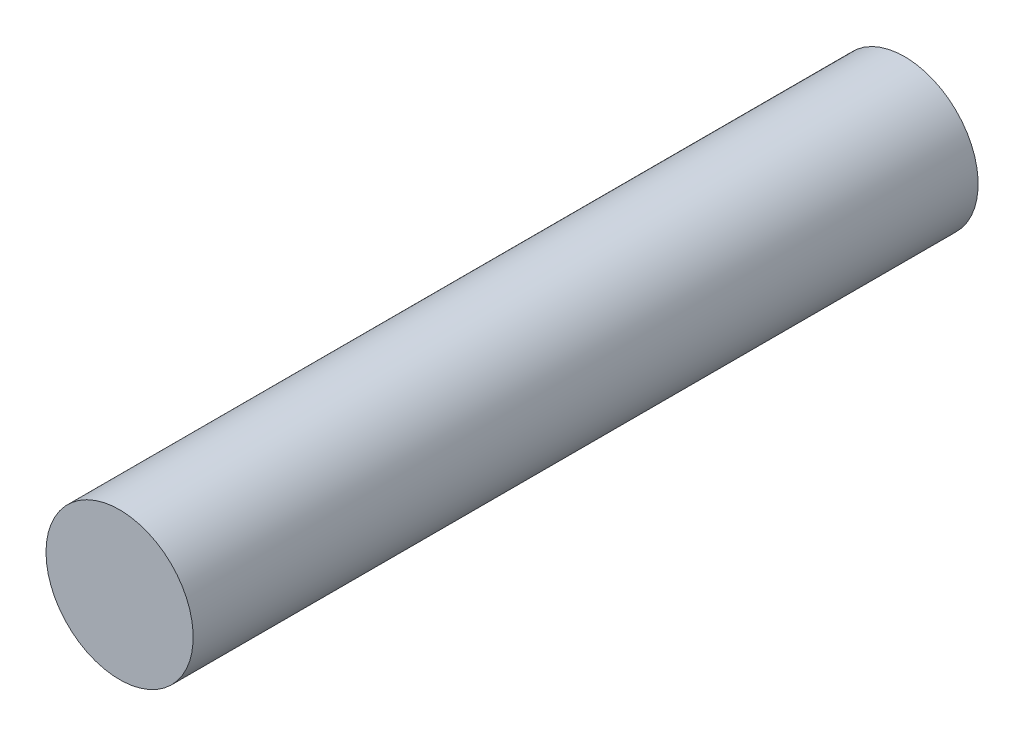
SolidWorks part; units mm, degrees
ref_plane "Front Plane" through (0, 0, 0) normal (0, 0, 1) x (1, 0, 0)
ref_plane "Top Plane" through (0, 0, 0) normal (0, 1, 0) x (1, 0, 0)
ref_plane "Right Plane" through (0, 0, 0) normal (1, 0, 0) x (0, 0, -1)
other "Configuration Table"
sketch "Sketch1" plane through (0, 0, 0) normal (0, 0, 1) x (1, 0, 0)
  circle A0 centre (70, -13) radius 15
extrude "Boss-Extrude1" add sketch "Sketch1" against normal blind 140 and the other way blind 20
